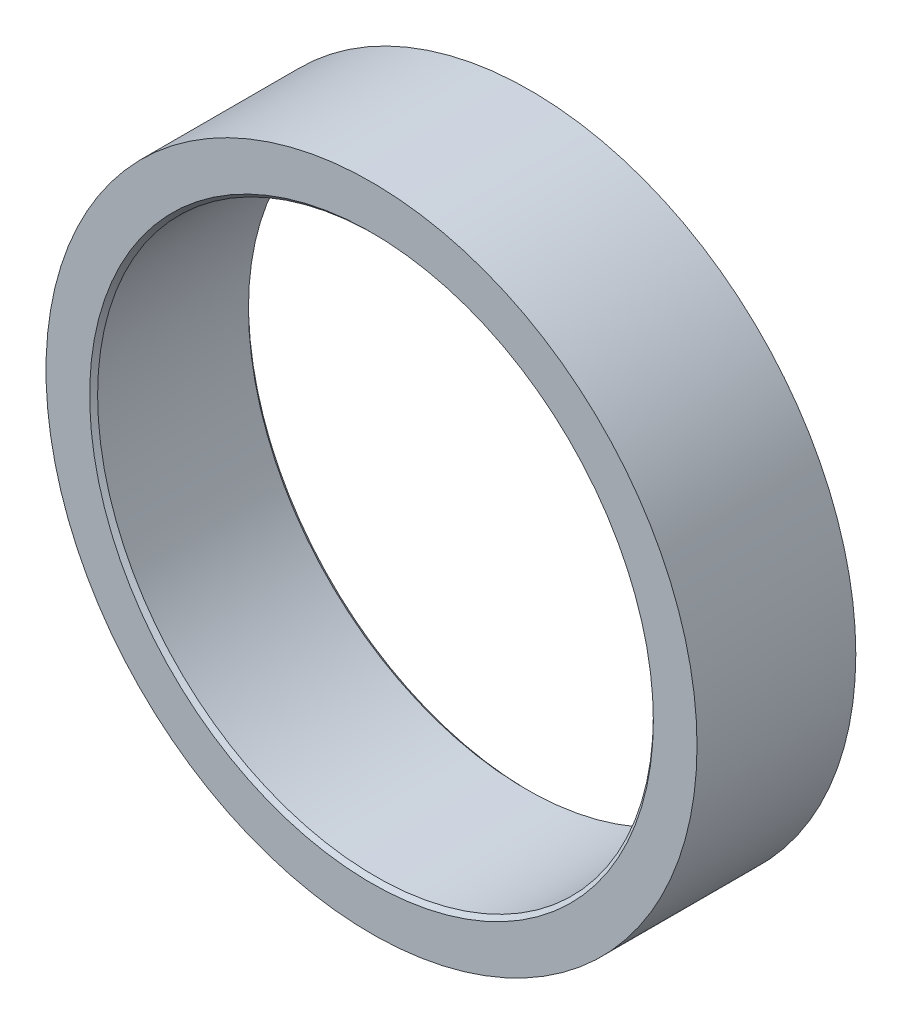
SolidWorks part; units mm, degrees
ref_plane "Front Plane" through (0, 0, 0) normal (0, 0, 1) x (1, 0, 0)
ref_plane "Top Plane" through (0, 0, 0) normal (0, 1, 0) x (1, 0, 0)
ref_plane "Right Plane" through (0, 0, 0) normal (1, 0, 0) x (0, 0, -1)
sketch "Sketch1" plane through (0, 0, 0) normal (0, 0, 1) x (1, 0, 0)
  circle A0 centre (0, 0) radius 35
  circle A1 centre (0, 0) radius 41
  dimension "D1" = 70
  dimension "D2" = 82
extrude "Boss-Extrude1" add sketch "Sketch1" along normal blind 20
chamfer "Chamfer1" distance 0.5 angle 45 2 edges at (35, 0, 20) (35, 0, 0)
